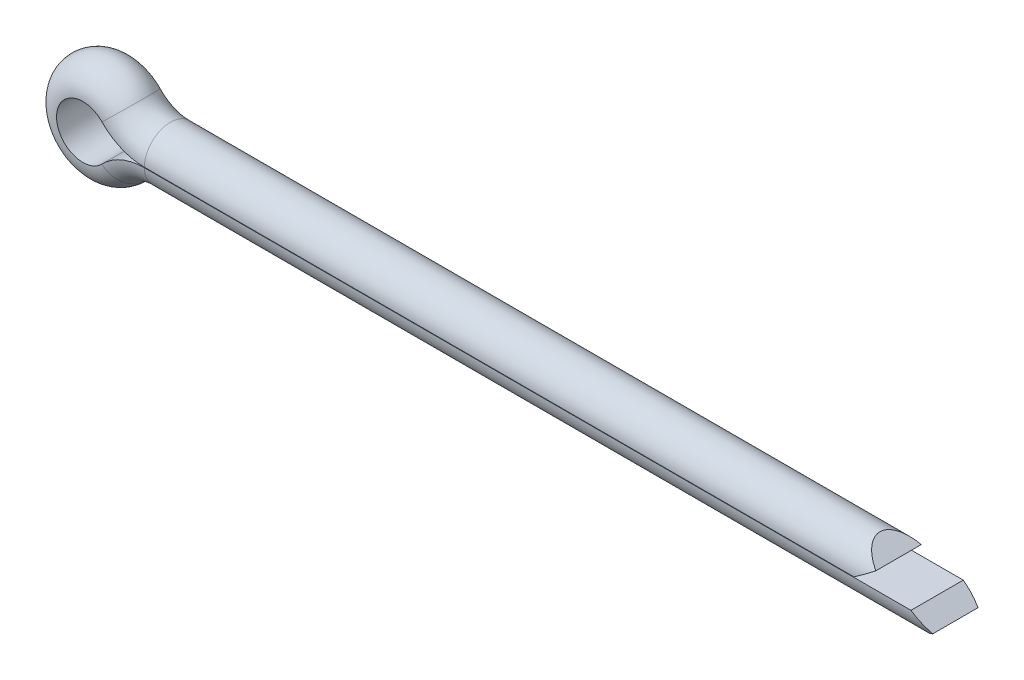
SolidWorks part; units mm, degrees
material "Q235"
ref_plane "Front Plane" through (0, 0, 0) normal (0, 0, 1) x (1, 0, 0)
ref_plane "Top Plane" through (0, 0, 0) normal (0, 1, 0) x (1, 0, 0)
ref_plane "Right Plane" through (0, 0, 0) normal (1, 0, 0) x (0, 0, -1)
sketch "Dimension sketch" plane through (0, 0, 0) normal (0, 0, 1) x (1, 0, 0)
  line L0 (34.7, 1.15) -> (2.7, 1.15)
  line L1 (2.7, -1.15) -> (37.2, -1.15)
  line L2 (2.7, 0) -> (27.3859, 0) construction
  line L3 (2.7, 0) -> (2.7, -0.0723) construction
  line L4 (-2.3, 0) -> (-2.3, 18.8979) construction
  arc A0 (2.7, 1.15) -> (1.6584, 1.5936) centre (2.7, 2.5946) cw
  arc A1 (1.6584, 1.5936) -> (1.6584, -1.5936) centre (0, 0) ccw
  arc A2 (1.6584, -1.5936) -> (2.7, -1.15) centre (2.7, -2.5946) cw
  dimension "c" = 4.6
  dimension "d1" = 2.3
  dimension "b" = 5
  dimension "l" = 32
  dimension "a" = 2.5
ref_plane "Plane1" through (34.7, 1.15, 0) normal (-1, 0, 0) x (0, 0, 1)
sketch "Sketch2" plane through (34.7, 1.15, 0) normal (-1, 0, 0) x (0, 0, 1)
  line L0 (0, -3.45) -> (0, 1.15) construction
  line L1 (-1.15, -1.14) -> (1.15, -1.14)
  arc A0 (1.15, -1.14) -> (-1.15, -1.14) centre (0, -1.15) ccw
  dimension "d" = 2.3
  dimension "D1" = 0.01
sweep "Sweep2" add profiles "Sketch2" path "Dimension sketch"
sketch "Sketch3" plane through (0, 0, 0) normal (0, 0, 1) x (1, 0, 0)
  line L0 (2.7, 0) -> (2.7, 16.2682) construction
  line L1 (2.7, 0) -> (37.4999, 0) construction
  line L2 (37.2, -1.15) -> (37.2, -0.01) construction
  line L3 (34.7, 0.57) -> (33.8823, 1.15)
  line L4 (34.7, 1.15) -> (2.7, 1.15) construction
  line L5 (2.7, -1.15) -> (37.2, -1.15) construction
  line L6 (34.7, 0.57) -> (33.8753, 0)
  line L7 (37.2, -0.58) -> (36.3823, 0)
  line L9 (37.2, -0.58) -> (36.3753, -1.15)
  line L10 (36.3823, 0) -> (33.8753, 0)
  line L11 (33.8823, 1.15) -> (37.21, 1.15)
  line L12 (37.21, 1.15) -> (37.21, -1.15)
  line L13 (37.21, -1.15) -> (36.3753, -1.15)
  line L14 (34.7, 1.15) -> (34.7, 0.01) construction
  dimension "D1" = 0.01
  dimension "D3" = 70
  dimension "D4" = 70
extrude "Cut-Extrude1" cut sketch "Sketch3" against normal through all and the other way through all
